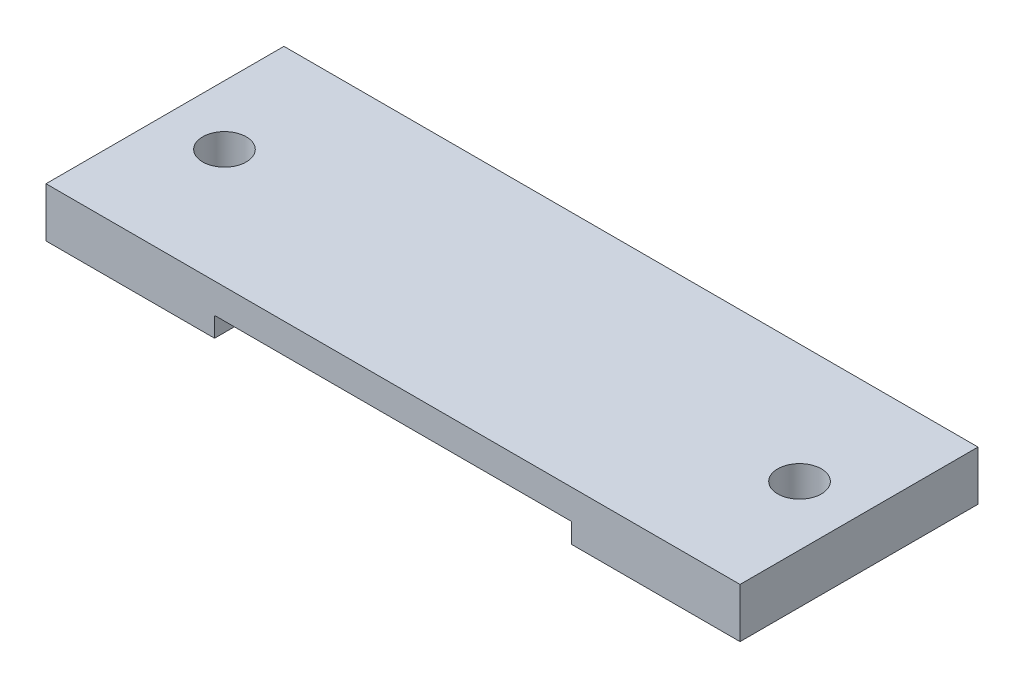
from build123d import *

# Parameters (mm, degrees)
SKETCH1_W           = 350
SKETCH1_H           = 120
BOSS_EXTRUDE1_DEPTH = 25
SKETCH2_W           = 180
SKETCH2_H           = 20
CUT_EXTRUDE1_DEPTH  = 214.658606192
SKETCH3_R           = 11
CUT_EXTRUDE2_DEPTH  = 25
FILLET1_R           = 0.5


with BuildPart() as part:
    # Sketch1 → Boss-Extrude1 (new body)
    with BuildSketch(Plane(origin=(0, 0, 0), x_dir=(1, 0, 0), z_dir=(0, 1, 0))):
        Rectangle(SKETCH1_W, SKETCH1_H)
    extrude(amount=BOSS_EXTRUDE1_DEPTH)

    # Sketch2 → Cut-Extrude1 (cut, through all)
    with BuildSketch(Plane.XY.offset(60)):
        Rectangle(SKETCH2_W, SKETCH2_H)
    extrude(amount=-CUT_EXTRUDE1_DEPTH, mode=Mode.SUBTRACT)

    # Sketch3 → Cut-Extrude2 (cut)
    with BuildSketch(Plane(origin=(0, 25, 0), x_dir=(1, 0, 0), z_dir=(0, 1, 0))):
        with Locations(Location((-145, 0, 0), (0, 0, 270))):
            Circle(SKETCH3_R)
        with Locations(Location((145, 0, 0), (0, 0, 90))):
            Circle(SKETCH3_R)
    extrude(amount=-CUT_EXTRUDE2_DEPTH, mode=Mode.SUBTRACT)

    # Fillet1
    fillet1_edges = [part.edges().sort_by_distance(p)[0] for p in [
        (90, 10, 0),
        (-90, 10, 0),
    ]]
    fillet(fillet1_edges, radius=FILLET1_R)


solid = part.part
